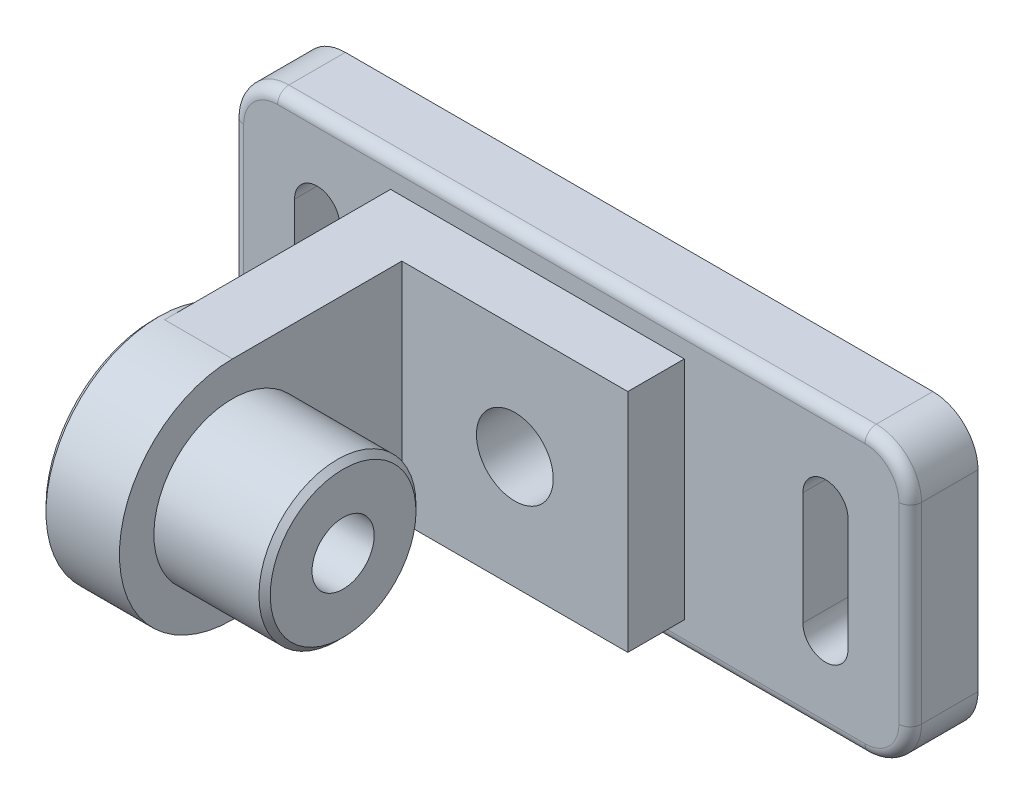
SolidWorks part; units mm, degrees
ref_plane "Front Plane" through (0, 0, 0) normal (0, 0, 1) x (1, 0, 0)
ref_plane "Top Plane" through (0, 0, 0) normal (0, 1, 0) x (1, 0, 0)
ref_plane "Right Plane" through (0, 0, 0) normal (1, 0, 0) x (0, 0, -1)
other "Configuration Table"
sketch "Sketch1" plane through (0, 0, 0) normal (0, 0, 1) x (1, 0, 0)
  line L0 (-22.5, 5) -> (-22.5, -5) construction
  line L1 (-26, 12.5) -> (26, 12.5)
  line L2 (-30, 8.5) -> (-30, -8.5)
  line L3 (-26, -12.5) -> (26, -12.5)
  line L4 (30, 8.5) -> (30, -8.5)
  line L5 (-30, 12.5) -> (30, -12.5) construction
  line L6 (-30, -12.5) -> (30, 12.5) construction
  line L7 (-20.5, 5) -> (-20.5, -5)
  line L8 (-24.5, 5) -> (-24.5, -5)
  line L9 (0, 0) -> (0, 12.5) construction
  line L10 (22.5, 5) -> (22.5, -5) construction
  line L11 (20.5, 5) -> (20.5, -5)
  line L12 (24.5, 5) -> (24.5, -5)
  line L13 (0, 0) -> (-30, 0) construction
  circle A0 centre (0, 0) radius 3.4
  arc A1 (-20.5, 5) -> (-24.5, 5) centre (-22.5, 5) ccw
  arc A2 (-24.5, -5) -> (-20.5, -5) centre (-22.5, -5) ccw
  arc A3 (20.5, 5) -> (24.5, 5) centre (22.5, 5) cw
  arc A4 (24.5, -5) -> (20.5, -5) centre (22.5, -5) cw
  arc A5 (-30, -8.5) -> (-26, -12.5) centre (-26, -8.5) ccw
  arc A6 (26, -12.5) -> (30, -8.5) centre (26, -8.5) ccw
  arc A7 (26, 12.5) -> (30, 8.5) centre (26, 8.5) cw
  arc A8 (-26, 12.5) -> (-30, 8.5) centre (-26, 8.5) ccw
  point P0 (0, 0)
  point P10 (-22.5, 0)
  point P18 (22.5, 0)
  dimension "D4" = 2
  dimension "D5" = 6.8
  dimension "D7" = 4
  dimension "D1" = 60
  dimension "D2" = 25
  dimension "D3" = 10
  dimension "D6" = 45
extrude "Boss-Extrude1" add sketch "Sketch1" along normal blind 6
chamfer "Chamfer1" distance 1 angle 45 1 edges at (3.4, 0, 0)
sketch "Sketch2" plane through (0, 0, 6) normal (0, 0, 1) x (1, 0, 0)
  line L1 (-16, 10) -> (-10, 10)
  line L2 (-16, 10) -> (-16, -10)
  line L3 (-16, -10) -> (-10, -10)
  line L4 (-10, 10) -> (-10, -10)
  dimension "D1" = 10
  dimension "D2" = 6
  dimension "D3" = 20
  dimension "D4" = 10
extrude "Boss-Extrude2" add sketch "Sketch2" along normal blind 30
sketch "Sketch3" plane through (-16, 0, 0) normal (-1, 0, 0) x (0, 0, 1)
  line L0 (36, 10) -> (36, -10) construction
  line L1 (36, -10) -> (6, -10) construction
  line L2 (26, 10) -> (26.3945, 15.3085)
  line L3 (26.3945, 15.3085) -> (43.3336, 9.2713)
  line L4 (43.3336, 9.2713) -> (37.7068, -17.6906)
  line L5 (37.7068, -17.6906) -> (26, -10)
  arc A0 (26, -10) -> (26, 10) centre (26, 0) ccw
  circle A1 centre (26, 0) radius 2.75
  dimension "D1" = 20
  dimension "D3" = 5.5
  dimension "D2" = 10
extrude "Cut-Extrude1" cut sketch "Sketch3" against normal through all both and the other way through all
sketch "Sketch4" plane through (-16, 0, 0) normal (-1, 0, 0) x (0, 0, 1)
  circle A0 centre (26, 0) radius 2.75
  circle A1 centre (26, 0) radius 10
extrude "Boss-Extrude3" add sketch "Sketch4" along normal mid plane 2
chamfer "Chamfer2" distance 0.5 angle 45 1 edges at (-17, -10, 26)
fillet "Fillet1" radius 1 8 edges at (-28.8284, 11.3284, 6) (0, 12.5, 6) (28.8284, 11.3284, 6) (30, 0, 6) (28.8284, -11.3284, 6) (0, -12.5, 6) (-28.8284, -11.3284, 6) (-30, 0, 6)
sketch "Sketch5" plane through (0, 0, 6) normal (0, 0, 1) x (1, 0, 0)
  line L5 (10, -10) -> (-10, -10)
  line L6 (10, -10) -> (10, 10)
  line L7 (10, 10) -> (-10, 10)
  line L8 (-10, -10) -> (-10, 10)
  line L9 (10, -10) -> (-10, 10) construction
  line L10 (10, 10) -> (-10, -10) construction
  circle A2 centre (0, 0) radius 3.4
extrude "Boss-Extrude4" add sketch "Sketch5" along normal blind 5
sketch "Sketch6" plane through (-17, 0, 0) normal (-1, 0, 0) x (0, 0, 1)
  line L1 (28.3697, 4.0985) -> (23.6355, 4.1015)
  line L2 (23.6355, 4.1015) -> (21.2657, 0.003)
  line L3 (21.2657, 0.003) -> (23.6303, -4.0985)
  line L4 (23.6303, -4.0985) -> (28.3645, -4.1015)
  line L5 (28.3645, -4.1015) -> (30.7343, -0.003)
  line L6 (30.7343, -0.003) -> (28.3697, 4.0985)
  circle A0 centre (26, 0) radius 4.1 construction
  dimension "D1" = 8.2
extrude "Cut-Extrude2" cut sketch "Sketch6" against normal blind 3 and the other way through all
sketch "Sketch7" plane through (-10, 0, 0) normal (1, 0, 0) x (0, 0, -1)
  circle A0 centre (-26, 0) radius 2.75
  circle A1 centre (-26, 0) radius 6.95
  dimension "D1" = 13.9
extrude "Boss-Extrude5" add sketch "Sketch7" along normal blind 9.8
chamfer "Chamfer4" distance 0.5 angle 45 1 edges at (-0.2, 6.95, 26)
